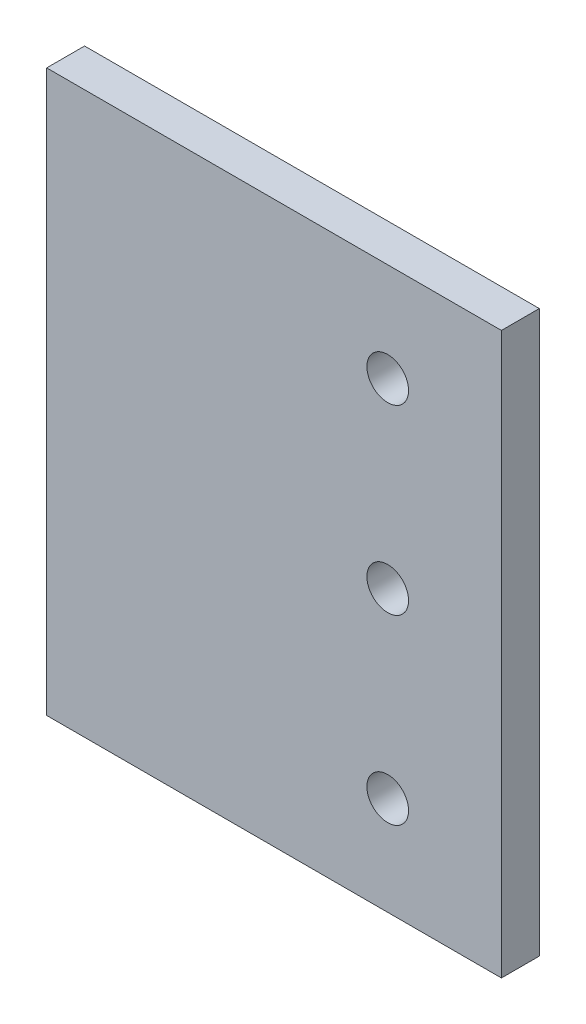
from build123d import *

# Parameters (mm, degrees)
SKETCH1_W           = 300
SKETCH1_H           = 370
SKETCH1_R           = 13.75
BOSS_EXTRUDE1_DEPTH = 25


with BuildPart() as part:
    # Sketch1 → Boss-Extrude1 (new body)
    with BuildSketch(Plane.XY):
        with Locations((150, 185)):
            Rectangle(SKETCH1_W, SKETCH1_H)
        with Locations((225, 305)):
            Circle(SKETCH1_R, mode=Mode.SUBTRACT)
        with Locations((225, 185)):
            Circle(SKETCH1_R, mode=Mode.SUBTRACT)
        with Locations((225, 65)):
            Circle(SKETCH1_R, mode=Mode.SUBTRACT)
    extrude(amount=BOSS_EXTRUDE1_DEPTH)


solid = part.part
